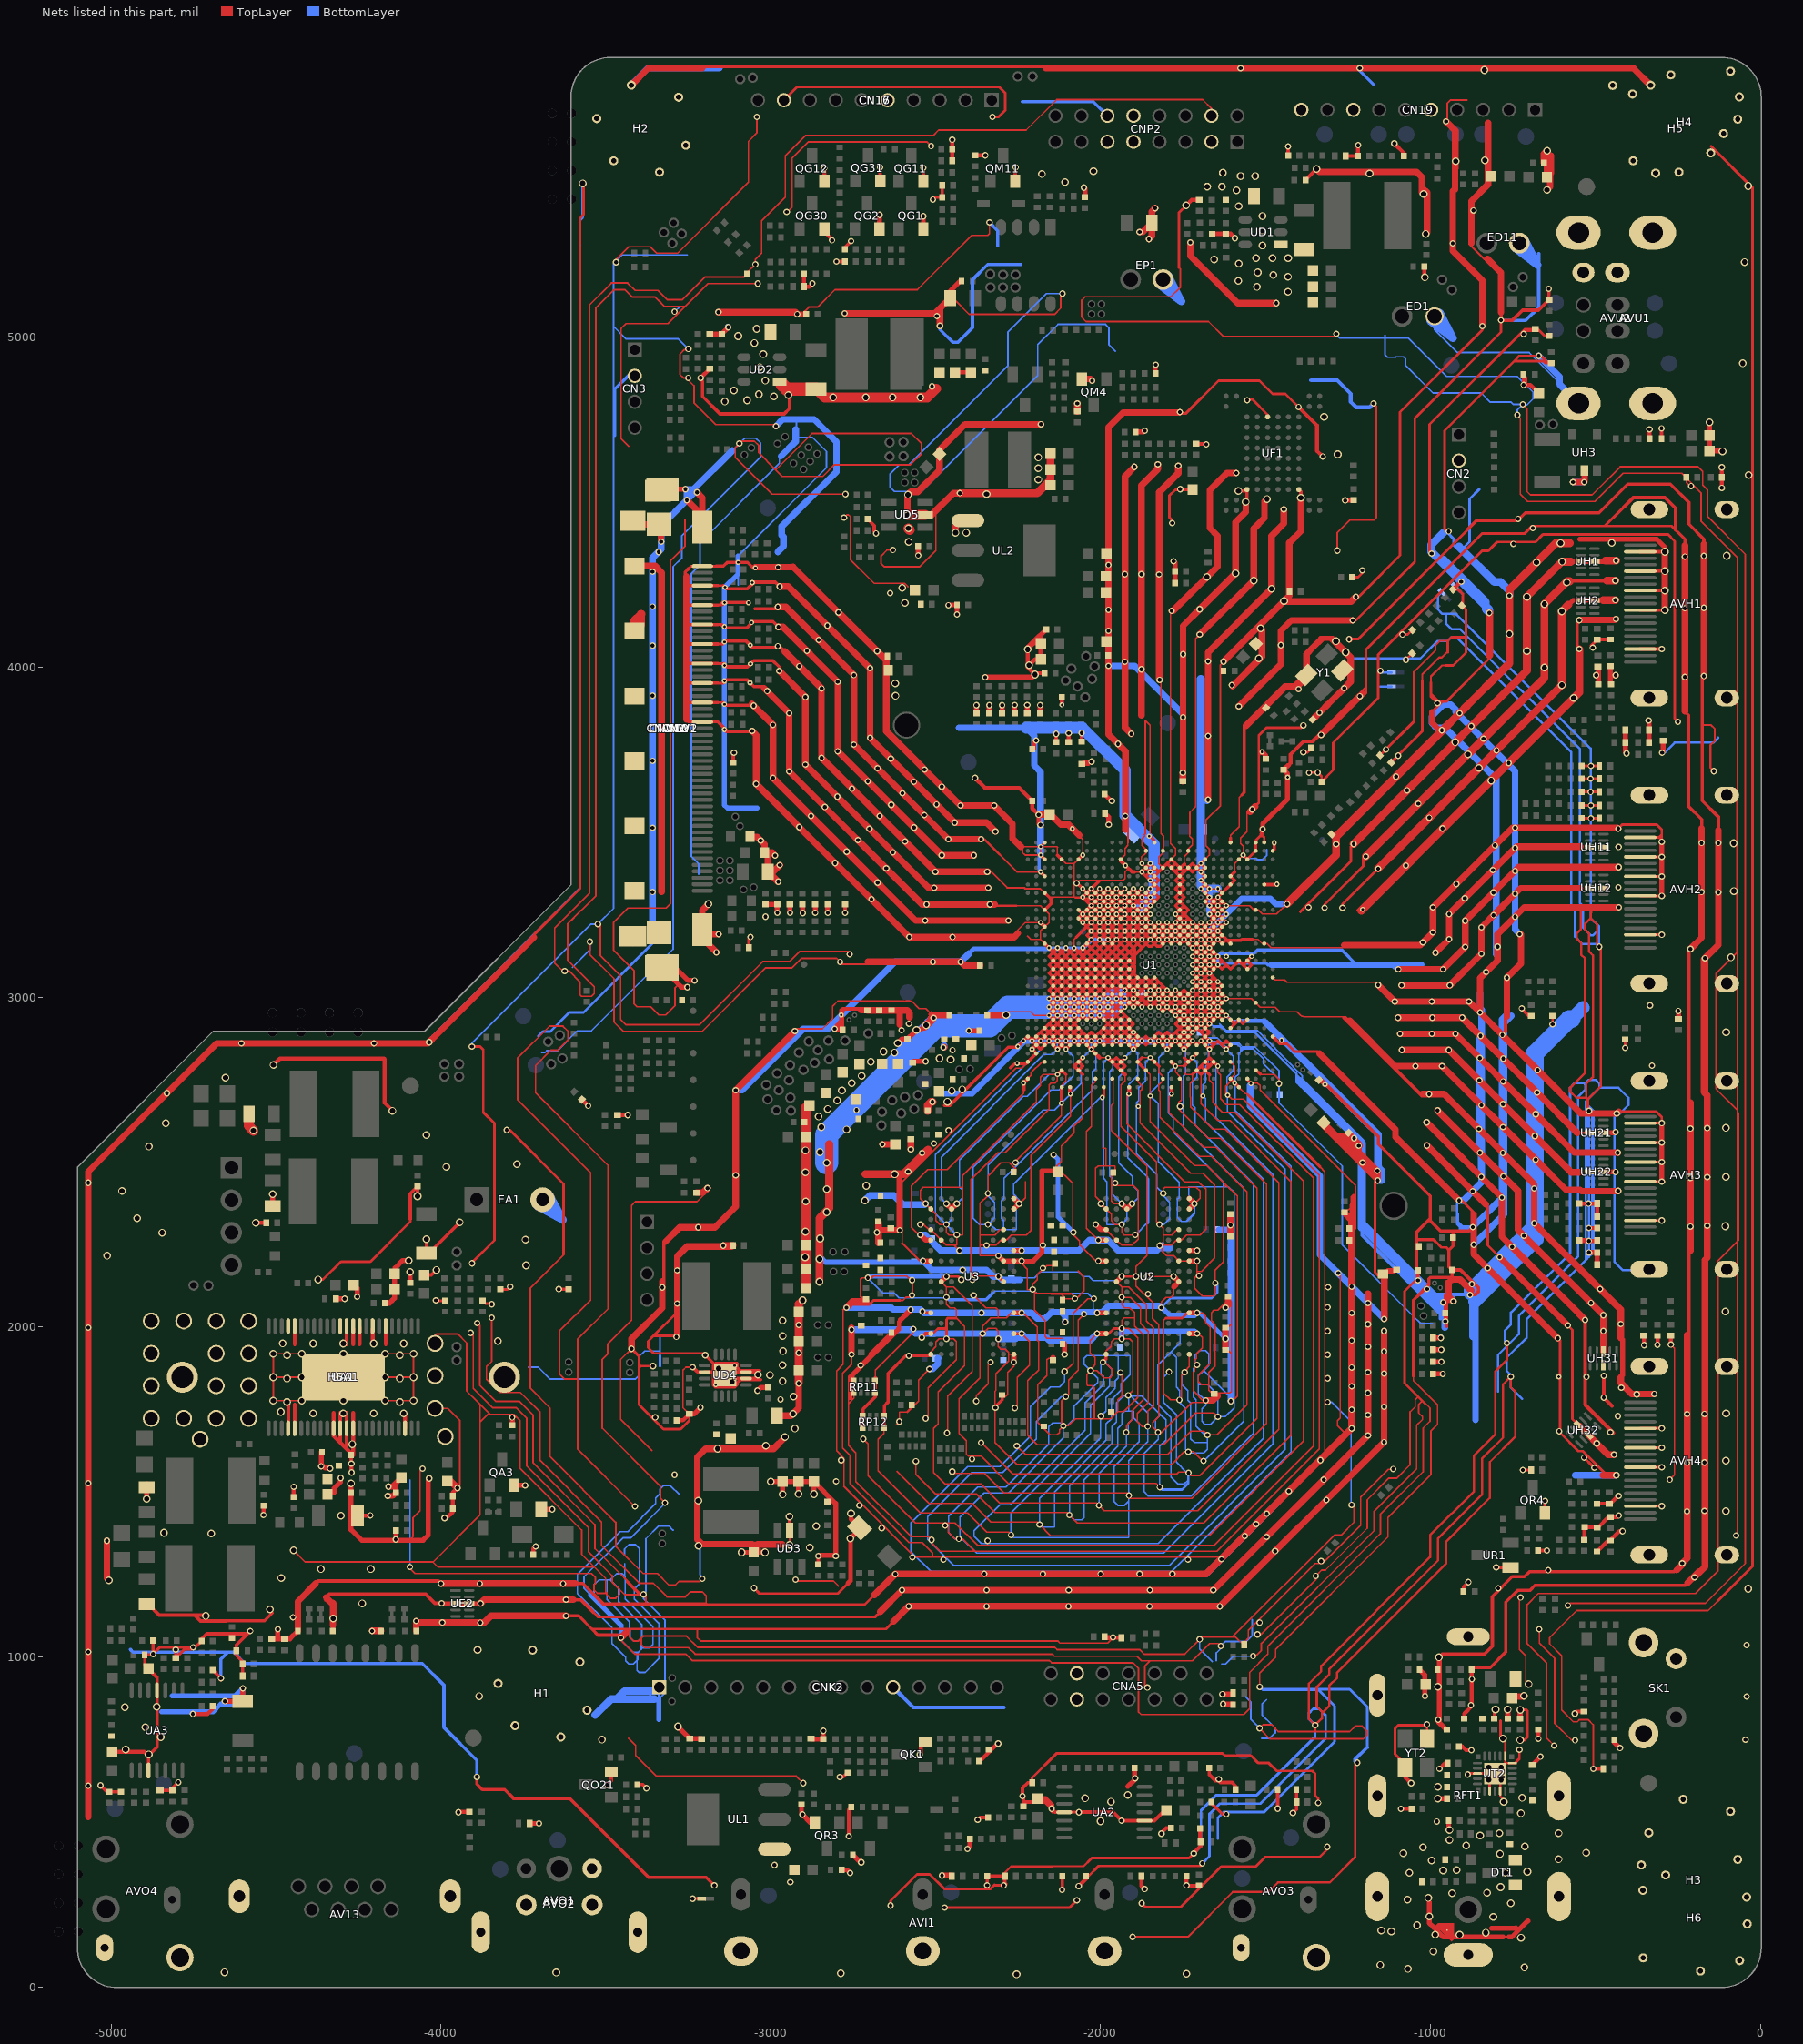
[diagram p0: the nets of this part, all layers, seen from the top]
# Altium PCB MISC86290.PcbDoc (part 15 of 31)
Units mil, origin at the board's own origin, x right, y up, seen from the top; angles counter-clockwise.
Board outline 5104.71 x 5851.49 mil, 2 copper layers (TopLayer, BottomLayer), stack 61.855 mil thick; 1026 components, 667 nets, 4280 pads, 2294 vias.

## Via types
v1: diameter 19.68, hole 11.81, TopLayer to BottomLayer, tented both sides, 1189 vias
v2: diameter 19.68/19.68 (per signal layer), hole 11.81, TopLayer to BottomLayer, tented both sides, 366 vias
v3: diameter 15.75, hole 7.87, TopLayer to BottomLayer, tented both sides, 348 vias
v4: diameter 23.62, hole 15.75, TopLayer to BottomLayer, tented both sides, 309 vias
v5: diameter 15.75/15.75 (per signal layer), hole 7.87, TopLayer to BottomLayer, tented both sides, 59 vias
v6: diameter 24/24 (per signal layer), hole 16, TopLayer to BottomLayer, tented both sides, 23 vias

## Nets (pads, with @x,y where several pads share a name; then routed paths per layer and width w, separated by ;. In a path a pad name is that pad's centre, name@x,y a point inside that pad or via, vN(x,y) a via of type N, cw(c..) or ccw(c..) an arc to the next point about the centre after c; other vN are vias at no path point) (continued)
GND: (continued)
  TopLayer w5: v4(-4447,1323) -4411.66,1287.66 -4024.21,1287.66 ; -4096,1353.66 -4084.5,1365.16 -4084.5,1422.5 -4063.5,1443.5 -4063.5,1563 v1(-4056,1570.5) ; v1(-4094,1273) -4094,1268 -4078.66,1252.66 -3543.66,1252.66 -3531.66,1240.66 -3531.66,1222.82 -3536.34,1218.13 -3536.34,1202.82 -3526.18,1192.66 -3497.82,1192.66 -3497,1193.47 ; pad.VIA5@-4037,1954 -4012,1979 -3949.14,1979 -3922,1951.86 -3922,1806.15 -3889.93,1774.07 ; -4025.22,2884.5 -4014.61,2884.5 ; pad.VIA5@-4018,1753.43 -3979.42,1753.43 -3942.5,1716.5 -3942.5,1519.5 v1(-3950,1512) ; v1(-3909.99,1981.99) -3902,1974 -3902,1814.43 -3842.57,1755 -3771.28,1755 -3740.5,1724.22 -3740.5,1579.78 -3553.25,1392.53 -3553.25,1318.82 -3481,1246.57 -3481,1226.53 -3443,1188.53 v1@-3390.49,1188.53 ; v1(-3890,2012) -3882,2004 -3882,1822.72 -3834.28,1775 -3763,1775 -3720.5,1732.5 -3720.5,1588.07 -3533.25,1400.82 -3533.25,1328.3 -3451.5,1246.55 ; -3881.5,1712 -3858.5,1735 -3850.85,1735 ; v1(-3846,2028) -3846,1896 -3862,1880 -3862,1842 -3821.48,1801.48 -3759.48,1801.48 -3699.91,1741.91 -3699.91,1595.76 -3513.25,1409.1 -3513.25,1337.62 -3399.13,1223.5 -3356.78,1223.5 -3315.28,1182 -3259,1182 -3244.16,1196.84 -3207.32,1196.84 -3196,1185.53 -3196,1159.5 ; -3628.15,2238 -3628.15,2218.85 -3728.8,2118.2 -3728.8,1813.96 -3668.84,1754 -3668.84,1606.58 -3470,1407.73 -3470,1335.5 -3387,1252.5 -3343.78,1252.5 -3308.78,1217.5 -3289.5,1217.5 -3278.5,1228.5 -3216.5,1228.5 v1(-3208,1237) ; -3596.55,3241.05 -3616.16,3221.43 ; -3587,1842 -3624.89,1842 -3641,1858.11 -3641,1987.14 -3546.25,2081.89 -3546.25,2467.99 -3768,2689.75 -3768,2815.06 -3671.06,2912 -3630,2912 -3615,2897 -3615,2869.61 -3645.11,2839.5 -3665.78,2839.5 -3713,2792.28 -3713,2709.7 -3493.25,2489.95 -3493.25,2055.67 -3586,1962.92 -3586,1630 v1(-3412,1456) ; -3579.11,5278.5 -3579.11,5283.17 ; v1@-3546.75,3168.12 v1@-3548.12,3168.12 ; v1@-3544.5,3164.5 v1@-3548.12,3168.12 ; -3535.37,1272.66 -4009.21,1272.66 -4024.21,1287.66 ; v1(-3524.48,3221.42) -3518.42,3221.42 -3517.13,3220.13 -3517.13,3126.42 -3455.34,3064.63 -3455.34,2932.06 -3439.28,2916 -3216.22,2916 -3024.38,3107.84 -2943.53,3107.84 -2913.37,3138 -2765,3138 v1@-2757,3130 ; -3477,1223 -3458,1204 -3458,1190 -3470,1178 -3487,1178 -3497,1188 -3497,1193.47 ; v1(-3469,5228) -3469,5236.5 -3430.5,5275 -3366,5275 -3346.84,5255.84 -3282.29,5255.84 -3068,5470.13 -3068,5594.07 -3042.5,5619.57 v1(-3042.5,5668.27) ; -3463.25,1065 -3462.25,1066 -3460.25,1068 -3444.25,1068 ; v1(-3454.25,1058) -3454.25,1050.22 -3412.18,1008.16 -3257.78,1008.16 -3237.94,988.31 ; -3454.11,5026.92 -3454.11,4692.61 -3431,4669.5 ; -3453.61,5027.42 -3438.92,5042.1 -3312.18,5042.1 -3259.78,5094.5 ; -3441.34,1236.39 -3451.5,1246.55 ; -3432,753.5 -3410.05,731.55 -3410.05,701.36 -3346.87,638.18 -2922.68,638.18 v1(-2901.5,617) ; -3431,1084.5 -3429.28,1082.77 -3429.28,1061.25 -3416.18,1048.16 -3401.82,1048.16 -3392.84,1057.13 ; v1@-3422.75,1934.25 -3455.5,1901.5 -3455.5,1720.5 -3361,1626 ; CNW3.52@-3418.3,3156.32 CNW3.52@-3418.3,3184.61 ; -3415,2999.86 -3415,3011.5 ; -3380.94,1159.5 -3378.75,1161.69 -3378.75,1182 v1(-3386.09,1189.34) v1@-3393.26,1189.34 ; -3332.75,5104.75 -3350.34,5122.34 ; -3332.36,5132.64 -3342.06,5142.34 ; v1(-3321,1467) -3334,1480 -3334,1516.27 -3511,1693.27 -3511,1901.86 -3495,1917.86 -3495,1947.85 -3422.25,2020.61 -3422.25,2368.75 -3411,2380 -3224,2380 -3191,2413 -3191,2420 v1(-3192,2421) ; -3279.89,3038.89 -3291,3027.79 -3291,2974 -3319,2946 -3339.79,2946 -3364.48,2970.68 -3405.68,2970.68 -3415,2980 -3415,3011.5 ; -3266.25,1778.5 -3266.25,1755.27 ; -3260,4446.95 -3260,4367.5 -3303.5,4324 -3303.5,3283.81 -3317.31,3270 -3432.86,3270 -3477.13,3225.72 -3477.13,3142.99 -3415,3080.86 -3415,3011.5 ; v1@-3250.5,4875 v1(-3250.5,4877.5) ; v1@-3248,4964 -3249,4963 -3262.08,4963 -3275.5,4949.58 -3275.5,4888 -3265,4877.5 v1(-3250.5,4877.5) ; CD34.1@-3247.25,1736.27 -3266.25,1755.27 ; -3222.5,1084.5 -3223.25,1083.75 -3223.25,1058.47 -3213.09,1048.31 ; -3215.64,1050.86 -3213.09,1048.31 ; UD4.6@-3201,1863.53 -3217.56,1863.53 -3232.03,1878 v1(-3237.25,1878) -3257.5,1878 -3266.25,1869.25 -3266.25,1755.27 ; -3195.5,988.31 -3237.94,988.31 ; v1@-3096.64,4677.06 -3107.81,4665.88 -3107.81,4636.57 -2995.91,4524.66 -2811,4524.66 ; v1@-3094.5,4678.5 -3094.5,4679.5 -3088.5,4685.5 -3064,4685.5 ; -3075.11,4685.5 -3064,4685.5 ; v1(-3039.34,5163.34) -3190.94,5163.34 -3259.78,5094.5 ; v1(-2984.5,4731) -2989.5,4736 -3167.5,4736 -3233,4801.5 -3233,4853.74 -3250.5,4871.24 v1(-3250.5,4877.5) ; v1(-2951.93,5380.19) -2949.81,5380.19 -2936.34,5393.66 -2936.34,5541.88 -2885.38,5592.85 -2527.35,5592.85 v1(-2514.5,5580) ; v4(-2943.25,1339.75) UD3.2@-2943.25,1383.12 ; v1(-2927.12,2897.12) -2920.25,2904 -2843.81,2904 -2812.66,2935.15 -2812.66,2972.34 -2797,2988 -2759.81,2988 ; v1(-2925.25,1234) -2921.16,1229.91 -2810.41,1229.91 -2795.5,1215 ; v1(-2920,5070.5) -2906.5,5070.5 -2885,5092 -2858.19,5092 -2805.19,5145 -2583,5145 ; v1(-2778.16,4453.64) -2769.8,4462 -2764.5,4462 -2760.52,4458.02 ; v1@-2777.25,4524.66 -2811,4524.66 ; v1(-2773.84,4524.66) -2811,4524.66 ; -2767.89,4708.85 -2759.25,4708.85 ; -2758.5,4456 -2758.5,4326.39 -2686.61,4254.5 -2594.5,4254.5 -2584.5,4244.5 ; -2757.5,5145 -2583,5145 ; -2740,2988 -2759.81,2988 ; v1(-2629.79,4355.5) -2648,4355.5 -2665.66,4337.84 -2665.66,4314.16 -2656,4304.5 -2607.5,4304.5 ; -2622.74,4304.5 -2607.5,4304.5 ; -2608.05,2080.53 -2599.72,2080.53 -2589.72,2090.53 -2577.7,2090.53 -2572.46,2095.77 v2(-2572.17,2096.06) ; -2584,3099.34 -2782.34,3099.34 v1(-2790,3107) -2801,3118 -2906.5,3118 -2935.66,3088.84 -3015.1,3088.84 -3207.94,2896 -3447.57,2896 -3475.34,2923.77 -3475.34,3056.35 -3548.82,3129.83 v1(-3548.82,3168.12) v1@-3548.12,3168.12 ; CL13.1@-2562.81,4234 CL13.1@-2557,4234 ; v6@-2546.97,2900.03 -2512.97,2934.03 -2512.97,2948.03 -2530.47,2965.53 -2550.95,2965.53 -2573.42,2988 -2759.81,2988 ; v2(-2546.57,2310.63) -2536.73,2310.63 -2520.98,2294.88 U3.D1@-2515.08,2294.88 ; v6@-2530,2914 v6(-2529.15,2914.85) ; -2499.64,4470.31 -2499.64,4353.89 -2549.03,4304.5 -2607.5,4304.5 ; -2475.18,3174.8 -2279.95,3174.8 -2272.65,3182.11 -2228.77,3225.98 v3(-2182.4,3225.98) U1.Y28@-2169.61,3213.19 ; CM17.2@-2456.28,5119 -2447.5,5119 -2398.5,5070 -2140,5070 -2121.25,5088.75 -2121.25,5128 v1(-2116.25,5133) ; UL2.1@-2419.27,4444.98 UL2.1@-2393.68,4444.98 ; v1(-2337.25,5348.75) -2337.25,5315 -2342.75,5309.5 -2391.13,5309.5 -2555.63,5145 -2583,5145 ; v6(-2286.72,2946.03) -2277.22,2955.53 -2212.22,2955.53 -2201.18,2944.49 v3(-2156.81,2944.49) ; v2(-2239.49,2200.39) v2@-2238.13,2199.03 ; -2229.32,3329.43 -2228.24,3328.35 -2182.4,3328.35 U1.AD28@-2169.61,3315.55 ; v1@-2080.04,3351 -2078.04,3353 -2047.2,3353 -2046.75,3353.45 ; -2063.98,3354.03 -1931.47,3354.03 -1926.4,3359.1 -1926.4,3379.67 -1915.77,3390.3 ; -2059.59,3482.89 -2057.72,3481.03 -2054.45,3478.02 v3(-2054.45,3430.71) ; -2044,982 -2075.35,982 ; v5(-2028.86,2842.13) v5@-2028.76,2842.03 ; v1@-1962,1058 -1978,1042 -2124,1042 -2130.31,1048.31 -3213.09,1048.31 ; U1.AH19@-1939.29,3417.91 v3@-1926.18,3404.8 ; v3@-1926.18,3328.03 U1.AD18@-1913.7,3315.55 ; -1917.22,3468.11 -1917.22,3739.01 ; -1905,3379.53 v3(-1875.32,3379.53) ; -1882,1022 -1881.09,1021.09 ; -1878,826 -1885.85,833.85 -1885.85,965.85 -1902,982 -2075.35,982 ; -1877.5,825.5 -1566.17,825.5 -1548.5,843.17 -1548.5,952.83 -1493,1008.33 -1493,1032.4 -1152.09,1373.31 -1152.09,1431.54 -1022.3,1561.33 -1022.3,1693.41 -1001.66,1714.06 ; -1867.22,3492.35 -1865,3494.57 -1865,3839.11 -1850.5,3824.61 -1850.5,3491 -1837.22,3477.72 U1.AK15@-1837.22,3471.77 ; v1(-1858.5,907) -1860,907 -1865.85,912.85 -1865.85,972.23 -1850.08,988 ; v3(-1853.25,3487.8) U1.AK15@-1837.22,3471.77 ; -1817.22,3506.05 -1817.22,4168.52 ; -1786.58,3464.02 -1788.22,3465.67 -1788.22,4163.14 -1774.21,4177.16 ; -1762.25,5211.58 -1758.5,5207.83 -1758.5,5152.36 -1787.7,5123.16 -2047.34,5123.16 -2057.75,5112.75 -2057.75,5061 -2044.91,5048.16 -1673.16,5048.16 -1628.5,5003.5 -1293.5,5003.5 v1(-1286,5011) ; -1729.72,3494.43 -1729.72,3560.23 -1712.22,3577.73 -1712.22,4086.78 v2(-1699.87,4099.13) ; v1@-1700,1057 v1(-1700,1053) ; U1.AH9@-1683.39,3417.91 -1670.59,3430.71 -1670.59,3449.3 -1680.43,3459.14 ; CNP2.4@-1664.51,5671.74 -1664.51,5694.51 -1691,5721 -2133.5,5721 -2226,5628.5 -2491,5628.5 -2506.65,5612.85 -2893.66,5612.85 -2956.34,5550.17 -2956.34,5424.66 -3028.09,5352.91 -3028.09,5255.13 -3047,5236.22 v1(-3047,5221.5) -3072.73,5195.77 DG11.A@-3072.73,5192 -3081.39,5183.34 -3199.23,5183.34 -3268.07,5114.5 -3314.22,5114.5 -3342.06,5142.34 ; -1637.22,3580.22 -1637.22,4007.78 v2(-1627.47,4017.53) ; v1(-1636,1033) -1643.61,1040.61 -1669.96,1040.61 -1722.57,988 -1850.08,988 ; v3@-1619.31,2995.77 -1542.73,2995.77 U1.L3@-1529.84,2982.87 ; U1.B6@-1606.68,2752.49 -1593.82,2765.35 -1593.82,2790.94 U1.D6@-1606.61,2803.74 ; U1.A5@-1581.02,2726.97 -1561.49,2707.43 -1556.76,2707.43 -1553.73,2704.4 ; v1(-1538,1002) -1531,1002 -1513,1020 -1513,1040.69 -1172.09,1381.6 -1172.09,1439.82 -1042.3,1569.61 -1042.3,1701.7 -1024.52,1719.48 -1024.52,1728.34 -1036.34,1740.17 -1036.34,1764.76 -1025.58,1775.53 ; v1@-1528,1068 v1(-1525,1068) -1513.86,1068 -1347.5,1234.36 v1(-1347.5,1245.5) -1330,1263 -1318.86,1263 -1192.01,1389.85 -1192.01,1475.92 -1125.93,1542 -1102,1542 -1062.22,1581.78 -1062.22,1742.6 -1046.66,1758.17 -1046.66,1779.34 -1036.78,1789.22 ; v1@-1523.91,784.09 v1(-1518.23,784.09) -1507.98,794.34 -1480.82,794.34 -1470.66,784.18 -1470.66,782.34 -1461.82,773.5 -1245.5,773.5 -1229,790 -1207.47,790 -1193.66,776.18 -1193.66,761.82 -1203.97,751.5 -1487.33,751.5 v1@-1513.83,778 ; v1(-1518.34,1103.84) -1528.73,1103.84 ; v1(-1518,909) -1518,950.81 -1470,998.81 -1470,1022.87 -1129.09,1363.79 -1129.09,1422.01 -999.3,1551.8 -999.3,1683.89 -978.66,1704.53 -978.66,1764.06 -1052,1837.41 -1052,1851 ; v1@-1513,907 v1@-1512.17,907.83 ; v1(-1331.84,1290.34) -1339.19,1283 ; v1@-1287.2,2164.6 -1273.72,2151.12 ; v1(-1279.86,2163.36) -1273.72,2157.22 -1273.72,2151.12 ; -1257.32,1674.32 -1257.32,1676.25 -1282.34,1701.28 -1282.34,1716.18 -1273.72,1724.8 -1273.72,2151.12 ; v1@-1242.66,1458.34 -1240.38,1460.62 v1(-1239.35,1460.62) -1232.01,1453.27 -1232.01,1408.08 -1270.09,1370 -1290.85,1370 -1600.24,1060.61 ; v1(-1173,4800) v1@-1168,4795 ; -1168,4658.89 v1@-1168,4795 ; RFT1.5@-1161.42,844.11 RFT1.5@-1161.42,883.86 ; v1(-1113.5,1569.5) -1112.5,1568.5 -1127.71,1568.5 -1212.01,1484.2 -1212.01,1398.46 -1327.47,1283 -1339.19,1283 ; -1079,1848.5 -1079,1831.88 -1001.66,1754.54 -1001.66,1714.06 ; -1001.66,1725.5 -1001.66,1714.06 ; v1(-953,5655) v1@-950.54,5657.46 ; v1@-949,5651 -949,5710.21 -939.82,5719.39 -889.39,5719.39 ; v1(-737.11,4764.63) -728,4755.53 -728,4525.28 -705.41,4502.7 -501.88,4502.7 -416.57,4588 -239,4588 DT2.A@-224.73,4573.73 ; v1(-727.5,1180) -730.5,1177 -730.5,1022 -711.28,1002.78 -711.28,925.88 v4(-702.7,917.3) ; v1(-720.28,4796.85) -708,4784.58 -708,4533.57 -697.13,4522.7 -510.16,4522.7 -424.86,4608 -189,4608 -174.91,4593.91 -174.91,4552.19 -160,4537.28 -160,4457 -46,4343 -46,1283.03 -166.53,1162.5 -577,1162.5 v2(-583.5,1156) ; v2@-670,1083 -670,1042.35 -624,996.35 -624,799 -571.5,746.5 -562.5,746.5 v1(-562,747) ; v1(-625.22,730.75) -648.5,754.03 -648.5,981.56 -707.84,1040.9 -707.84,1157.85 -673.45,1192.25 -196.75,1192.25 -129,1260 -129,2200.5 -70,2259.5 ; v1@-507,660.5 -507,711.78 -507,714.14 ; -507,725 -507,714.14 ; v1@-299.12,4055.12 v1(-299,4055) ; v2(-275,1537) -260.5,1551.5 -260.5,1935.5 v1(-271.5,1946.5) ; DT2.A@-224.73,4576 DT2.A@-224.73,4573.73 ; v1(-210,4549.33) -213.33,4549.33 -224.73,4560.73 DT2.A@-224.73,4573.73 ; -128.81,1169.81 -158.28,1140.34 -557.16,1140.34 -639,1058.5 -639,1039.63 -602.5,1003.13 -602.5,838.64 -567.32,803.46 -554.81,803.46 -548.45,809.82 -522.55,809.82 -507,794.27 -507,714.14 ; v1(-74,1368) -70,1372 -70,2259.5 ; AVH2.23@-71.5,3603 -71.5,3134.5 -134.5,3071.5 -134.5,2722 -70,2657.5 -70,2652.5 ; -4024.21,1287.66 -3881.5,1430.37 -3881.5,1765.65 -3889.93,1774.07 ; -3889.93,1774.07 -3850.85,1735 ; -3850.85,1735 -3779.57,1735 -3760.5,1715.93 -3760.5,1571.5 -3573.25,1384.25 -3573.25,1310.53 -3501,1238.28 -3501,1197.47 -3497,1193.47 ; -3616.16,3221.43 -3530.11,3307.48 -3530.11,5089.85 -3474.96,5145 -3442.47,5145 -3419.82,5122.34 -3350.34,5122.34 ; -3616.16,3221.43 -3616.16,3112.44 -3535.5,3031.78 -3535.5,3010.5 -3543.5,3002.5 -3573.5,3002.5 -3577.92,3006.92 -3577.92,3045.43 -3611.63,3079.14 v1(-3624.82,3079.14) -3631.14,3079.14 -3655.5,3103.5 -3655.5,3208.97 -3549.11,3315.36 -3549.11,5099.14 -3483.25,5165 -3434.19,5165 -3411.53,5142.34 -3342.06,5142.34 ; -3451.5,1246.55 -3450.47,1246.55 -3437,1233.08 ; -3437,1233.08 -3437,1226.32 -3400.02,1189.34 v1@-3393.26,1189.34 ; -3437,1233.08 v1@-3393.26,1189.34 ; -3392.84,1057.13 -3392.84,1038.32 -3382.68,1028.16 -3249.5,1028.16 -3229.66,1008.31 -2146.88,1008.31 -2140.57,1002 -1890.32,1002 -1876.32,988 -1850.08,988 ; -3392.84,1057.13 -3386.98,1063 -3256.06,1063 -3221.37,1028.31 -2138.6,1028.31 -2132.28,1022 -1882.04,1022 -1881.09,1021.05 -1868.04,1008 -1745,1008 v1(-1700,1053) ; -3350.34,5122.34 -3322.5,5094.5 -3259.78,5094.5 ; -3237.94,988.31 -2155.17,988.31 -2148.85,982 -2075.35,982 ; -3064,4685.5 -3049.89,4685.5 -3036.75,4672.35 -3036.75,4650.11 -2987.63,4601 ; -2987.63,4601 -2983.17,4601 -2875.32,4708.85 -2759.25,4708.85 ; -2987.63,4601 -2965.29,4578.66 -2842.34,4578.66 -2807.15,4613.85 -2577.15,4613.85 -2543,4648 -2543,4677.5 -2574.35,4708.85 -2759.25,4708.85 ; U1.AK15@-1837.22,3471.77 -1836.93,3471.48 U1.AK15@-1836.93,3469.09 -1837.22,3469.39 U1.AK15@-1837.22,3471.77 ; v1(-1700,1053) -1692.39,1060.61 -1600.24,1060.61 ; -1600.24,1060.61 -1592.05,1060.61 -1568.44,1037 DA2.A@-1565.27,1037 -1565.27,1043.87 -1552.69,1056.45 -1552.69,1079.88 -1528.73,1103.84 ; -1528.73,1103.84 -1349.57,1283 -1339.19,1283 ; -1282,4408.5 -1282.6,4407.89 v1(-1282.6,4353.87) -1282.6,4350.61 -1282,4350 -1282,4408.5 ; -1282,4408.5 -1243.36,4447.14 -1171,4447.14 -1164.25,4453.89 -1164.25,4791.25 v1@-1168,4795 ; DT2.A@-224.73,4573.73 -180,4529 -180,4443.04 -70,4333.04 -70,2652.5 ; -70,2259.5 -67,2262.5 -67,2649.5 -70,2652.5 ; -70,2259.5 -70,2652.5
  TopLayer w5.91: -2618.43,1704.33 v2@-2610.55,1712.2 ; -2601.69,2254.53 v2@-2547.56,2200.39 ; v2@-2118.43,1705.31 -2118.43,1776.18 ; -2019.02,1722.05 -2019.02,1814.57 ; U1.M7@-1632.2,3008.46 v3@-1619.25,2995.64
  TopLayer w6: -2398.27,3276.78 -2255.71,3276.78 ; v1(-2362.86,3479.11) -2353,3479.11 -2255.32,3381.43 ; CI1.1@-2344.27,334.99 -2300.96,334.99 -2272.95,363 ; v1(-2344,3380.11) -2332,3380.11 -2283.67,3331.78 -2231.67,3331.78 -2229.32,3329.43 ; -2139,365.84 -2145.7,365.84 ; -2039,378 -2051.16,365.84 -2145.7,365.84 ; -1050.5,3975.92 -1050.5,3985.79 -984.84,4051.44 -984.84,4067.39 -972.43,4079.8 -947.84,4079.8 ; -1025.5,3959 -1025.5,3978.26 -973.92,4029.84 -966,4029.84 -947.84,4048 ; -998.84,3955 -998.84,3972.39 -965.39,4005.84 -956,4005.84 ; -882.96,5305 -882.96,5282.96 -786.25,5186.26 -786.25,5170 ; -176.5,3825 -150,3825 -138.16,3813.16 -138.16,3777.72 -151.5,3764.38 -151.5,3697 ; -151.5,3714 -151.5,3697 ; v1(-141,3685) -151.5,3695.5 -151.5,3697 ; -2272.95,363 -2148.54,363 -2145.7,365.84 ; -2272.95,363 -2270.11,365.84 -2145.7,365.84
  TopLayer w7: -3195.18,1158.68 -2715.32,1158.68 -2685.75,1188.25 ; v3(-2182.4,3456.3) U1.AK28@-2169.61,3469.09 ; v2(-1903,151) -1735.81,151 -1599.31,287.5 -1491.5,287.5 -1462.5,316.5 -1305.1,316.5 -1229,392.6 -1229,672.44 v1(-1222.44,679) ; UA2.10@-1867.52,503.49 UA2.10@-1867.44,503.41 ; -1350,774.5 v1(-1350,793) ; v1(-1258.63,4505.84) v1@-1257.7,4506.77 ; v1(-1151.76,3989.5) v1@-1149.26,3987 ; v1(-1075,4023) CO52.1@-1055.83,4042.17 ; UT2.EPAD@-804.89,646.37 -789.15,630.62 -789.15,577.15 -778.18,566.19 v4(-778.18,560.77) ; v1(-768.38,1951.12) -768.38,1900.53 -804.34,1864.57 -804.34,1674.42 -868.28,1610.48 -868.28,1501.8 -1001.09,1369 -1001.09,1302.69 -1331.49,972.29 -1331.49,956.3 -1369.16,918.63 -1369.16,812.16 v1(-1350,793) ; v1@-756.34,1848.34 v1(-757,1849) ; v1@-630,2918 D41.A@-630,2943.27 ; -555.22,2589 UH21.GND@-516.47,2589 ; -538.34,3272 -544,3266.34 -544,3206 -556.34,3193.66 -556.34,3177.4 -543.34,3164.4 -543.34,3128.43 -532,3117.09 -532,2769.94 -577,2724.94 -577,2714 -558.29,2695.29 -528.46,2695.29 ; v1@-519.69,2647.5 v1(-519.69,2655) -523.23,2658.54 -523.23,2690.06 ; -513,3272 -513,3255.94 -514.34,3254.6 -514.34,3239.4 ; v1(-1350,793) -1329.66,813.34 -1329.66,834.16 ; -1329.66,834.16 -1323.9,834.16 -1307.66,850.4 -1307.66,912.25 -1283.49,936.42 -1283.49,952.41 -953.09,1282.8 -953.09,1349.11 -820.28,1481.92 -820.28,1590.6 -742.88,1668 -742.88,1803.94 -757,1818.06 v1(-757,1849) ; -1329.66,834.16 -1345,849.5 -1345,908.85 -1307.49,946.36 -1307.49,962.35 -977.09,1292.74 -977.09,1359.05 -844.28,1491.86 -844.28,1600.54 -780.34,1664.48 -780.34,1825.66 v1(-757,1849) ; -528.46,2695.29 -528.46,2736.71 -507.66,2757.51 -507.66,3126.69 -519.34,3138.37 -519.34,3192.4 -532.34,3205.4 -532.34,3221.4 -514.34,3239.4 ; -528.46,2695.29 -523.23,2690.06 ; -523.23,2690.06 -483.66,2729.63 -483.66,3147.66 v1(-489,3153) -495.34,3159.34 -495.34,3220.4 -514.34,3239.4
  TopLayer w7.8: v1(-887.66,643.27) -884.57,646.37 UT2.16@-858.04,646.37 UT2.EPAD@-804.89,646.37 -820.64,630.62 UT2.21@-820.64,593.22 ; v4@-773.4,745.16 -773.4,677.86 -744.2,677.86 -730.55,691.51 v1(-730.55,718.58)
  TopLayer w7.87: v2@-2772.23,2058.66 -2770.67,2060.23 -2770.58,2060.31 -2760.42,2060.31 -2752.55,2068.19 -2728.47,2068.19 ; C102.1@-2711.21,2078.03 -2721.05,2068.19 -2728.47,2068.19 ; -2687.38,2080.53 -2608.05,2080.53 ; -2609.3,2080.53 -2688.63,2080.53 -2700.97,2068.19 -2728.47,2068.19 ; -2585.63,1742.72 C103.1@-2564.96,1763.39 ; U3.P1@-2509.17,1979.92 -2493.43,1995.67 -2473.74,1995.67 ; v2(-2467.83,1964.17) -2467.83,2001.57 -2467.83,2023.23 -2463.9,2027.17 -2438.31,2027.17 ; v2(-2467.83,2153.15) -2432.4,2153.15 v2(-2422.56,2143.31) ; v5(-1995.39,2695.47) -1990.47,2700.39 U1.A21@-1990.47,2726.97 ; -1975.71,1979.92 -1959.96,1995.67 v2@-1940.28,1995.67 ; v2(-1936.34,2153.15) v2(-1893.03,2153.15) ; -1802.48,2027.17 -1753.27,2027.17 -1737.52,2042.91 U2.M9@-1731.61,2042.91 ; U1.T9@-1683.39,3110.83 -1682.4,3110.83 v3@-1670.59,3122.64 ; -1553.73,2704.4 -1334.55,2485.22